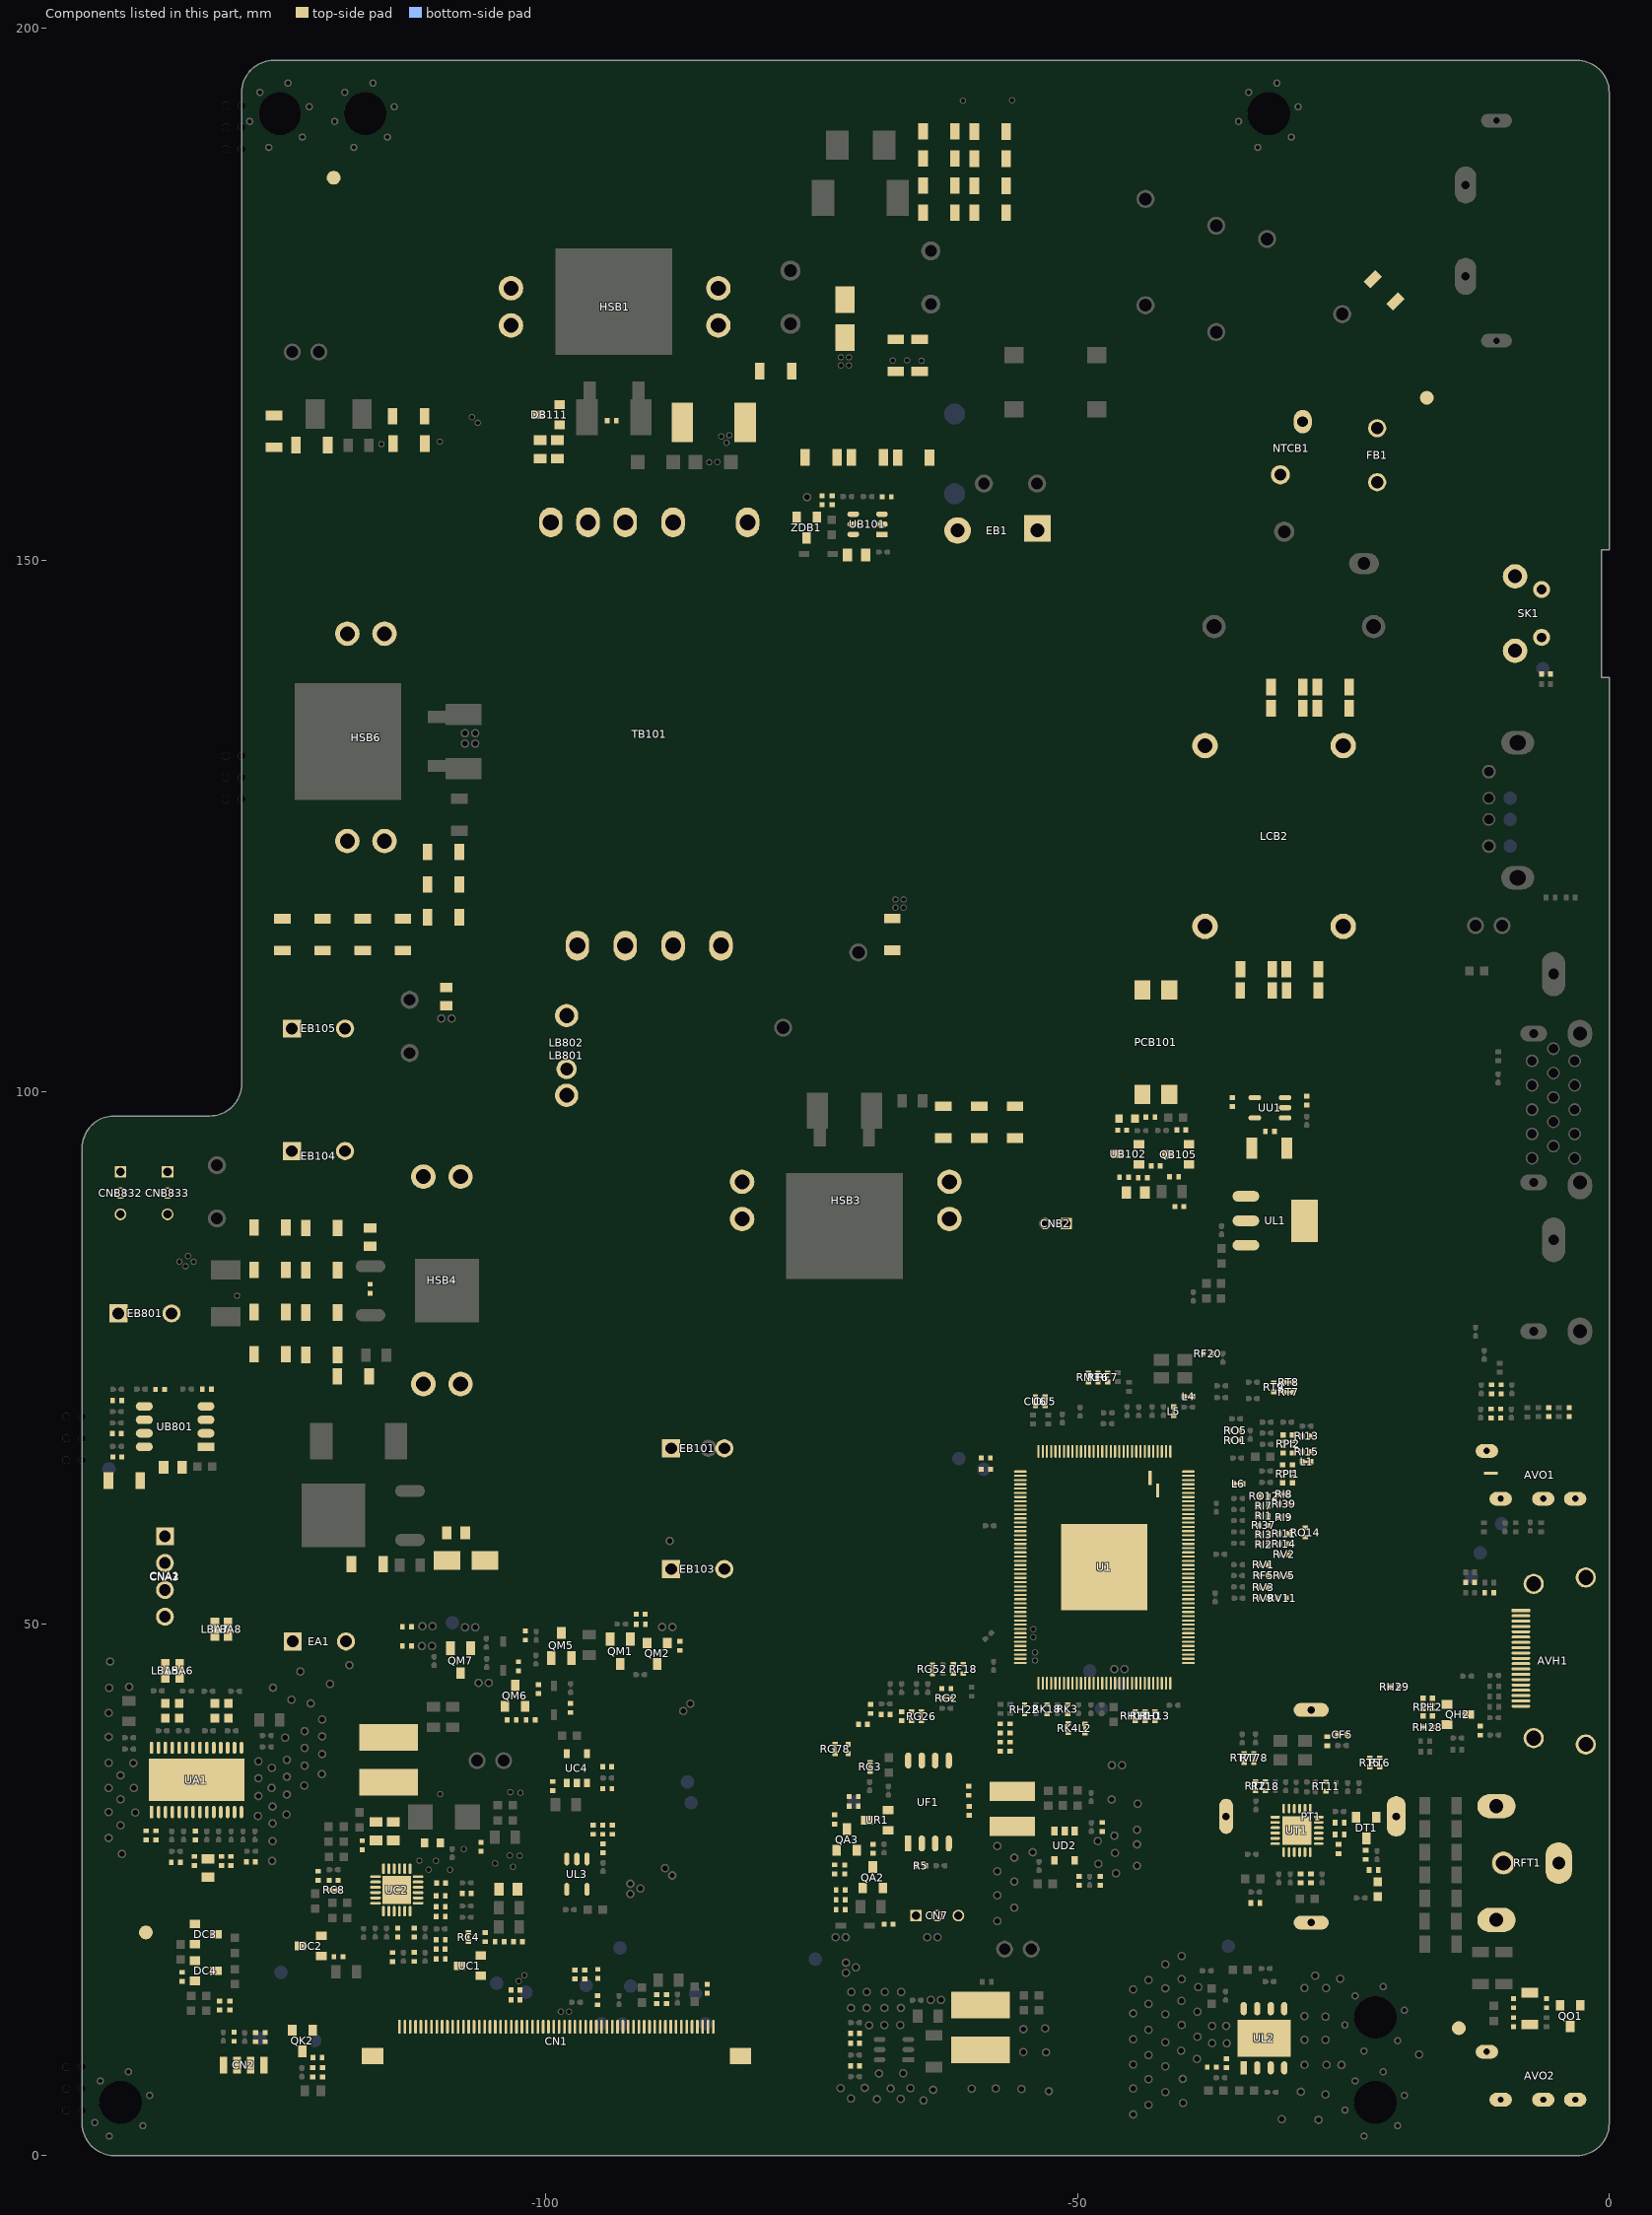
[diagram p0: the components of this part, seen from the top]
# Altium PCB MISC86383-9.PcbDoc (part 5 of 18)
Units mm, origin at the board's own origin, x right, y up, seen from the top; angles counter-clockwise.
Board outline 143.6 x 197 mm, 2 copper layers (TopLayer, BottomLayer), stack 1.571 mm thick; 743 components, 401 nets, 2996 pads, 1077 vias.
Unrouted connection lines stored in the file: 4.

## Footprints (in the part's own frame and the unit in brackets; to place one, negate y for a bottom-side part, rotate by r counter-clockwise, add the part's x,y. Pads: shape width x height; smd on the part's side, far side on the other; paste and mask are expansions set on the pad) (continued)
EC(10*12.5)-V-5#2 [mm] "机插5间距"
  round 0.5 on Keep-Out: 0(-0.75,0)
  rect 1.7x1.7 hole 1.1: 1(-2.5,0)
  rect 1.9x1.9 on Top Overlay: 1(-2.5,0)
  round 1.9 on Top Overlay: 1(2.5,0)
  round 1.7 hole 1.1: 2(2.5,0)
  BottomLayer lines w0.6: -2.92,-0.262 -2.89,-0.31 ; -2.92,-0.262 -2.991,-0.148 -4.056,1.556 ; -2.5,0 -2.627,0.127 -4.056,1.556 ; -2.19,0.39 -2.238,0.42 -2.42,0.534 -4.056,1.556 ; 2.19,-0.39 2.238,-0.42 ; 2.5,0 4.056,-1.556 ; 2.89,0.31 2.92,0.262 2.92,0.262 ; 2.238,-0.42 4.056,-1.556 ; 2.238,-0.42 2.238,-0.42 ; 2.238,-0.42 2.238,-0.42 ; 2.92,0.262 4.056,-1.556 ; 2.92,0.262 2.92,0.262
  silkscreen extent -5.2,-5.21 5.57,5.21, body extent -4.98,-4.99 5.01,4.99, height 14.01
EC(10*12.5)-V-5#3 [mm] "机插5间距"
  round 0.5 on Keep-Out: 0(-0.75,0)
  rect 1.7x1.7 hole 1.1: 1(-2.5,0)
  rect 1.9x1.9 on Top Overlay: 1(-2.5,0)
  round 1.9 on Top Overlay: 1(2.5,0)
  round 1.7 hole 1.1: 2(2.5,0)
  BottomLayer lines w0.6: -2.89,-0.31 -2.92,-0.262 -3.129,0.072 -4.056,1.556 ; -2.5,0 -2.78,0.28 -4.056,1.556 ; -2.19,0.39 -2.238,0.42 -2.5,0.584 -2.558,0.62 -2.754,0.742 -4.056,1.556 ; 2.19,-0.39 2.238,-0.42 ; 2.5,0 2.52,-0.02 2.704,-0.204 4.056,-1.556 ; 2.89,0.31 2.92,0.262 2.92,0.262 ; 2.238,-0.42 2.5,-0.584 2.52,-0.596 4.056,-1.556 ; 2.238,-0.42 2.238,-0.42 ; 2.238,-0.42 2.238,-0.42 ; 2.92,0.262 2.92,0.262 ; 2.92,0.262 3.016,0.108 4.056,-1.556
  silkscreen extent -5.2,-5.21 5.57,5.21, body extent -4.98,-4.99 5.01,4.99, height 14.01
EC(10*12.5)-V-5#4 [mm] "机插5间距"
  round 0.5 on Keep-Out: 0(0.025,-0.953)
  rect 1.7x1.7 hole 1.1: 1(-2.5,0)
  rect 1.9x1.9 on Top Overlay: 1(-2.5,0)
  round 1.9 on Top Overlay: 1(2.5,0)
  round 1.7 hole 1.1: 2(2.5,0)
  BottomLayer lines w0.6: -2.89,-0.31 -2.92,-0.262 -3.084,0 -4.056,1.556 ; -2.5,0 -4.056,1.556 ; -2.19,0.39 -2.238,0.42 -2.5,0.584 -4.056,1.556 ; 2.19,-0.39 2.238,-0.42 ; 2.5,0 4.056,-1.556 ; 2.89,0.31 2.92,0.262 2.92,0.262 ; 2.238,-0.42 4.056,-1.556 ; 2.238,-0.42 2.238,-0.42 ; 2.238,-0.42 2.238,-0.42 ; 2.92,0.262 4.056,-1.556 ; 2.92,0.262 2.92,0.262
  silkscreen extent -5.2,-5.21 5.57,5.21, body extent -4.98,-4.99 5.01,4.99, height 14.01
EC(10*12.5)-V-5#5 [mm] "机插5间距"
  round 0.5 on Keep-Out: 0(-0.75,0)
  rect 1.7x1.7 hole 1.1: 1(-2.5,0)
  rect 1.9x1.9 on Top Overlay: 1(-2.5,0)
  round 1.9 on Top Overlay: 1(2.5,0)
  round 1.7 hole 1.1: 2(2.5,0)
  BottomLayer lines w0.6: -2.89,-0.31 -2.92,-0.262 -3.182,0.157 -4.056,1.556 ; -2.5,0 -2.792,0.292 -4.056,1.556 ; -2.19,0.39 -2.238,0.42 -2.5,0.584 -4.056,1.556 ; 2.19,-0.39 2.238,-0.42 ; 2.5,0 4.056,-1.556 ; 2.89,0.31 2.92,0.262 2.92,0.262 ; 2.238,-0.42 4.056,-1.556 ; 2.238,-0.42 2.238,-0.42 ; 2.238,-0.42 2.238,-0.42 ; 2.92,0.262 4.056,-1.556 ; 2.92,0.262 2.92,0.262
  silkscreen extent -5.2,-5.21 5.57,5.21, body extent -4.98,-4.99 5.01,4.99, height 14.01
EC(10*12.5)-V-5#6 [mm] "机插5间距"
  round 0.5 on Keep-Out: 0(-0.75,0)
  rect 1.7x1.7 hole 1.1: 1(-2.5,0)
  rect 1.9x1.9 on Top Overlay: 1(-2.5,0)
  round 1.9 on Top Overlay: 1(2.5,0)
  round 1.7 hole 1.1: 2(2.5,0)
  BottomLayer lines w0.6: -2.89,-0.31 -2.92,-0.262 -3.084,0 -4.056,1.556 ; -2.5,0 -2.68,0.18 -4.056,1.556 ; -2.19,0.39 -2.238,0.42 -2.377,0.506 -2.5,0.584 -2.68,0.696 -4.056,1.556 ; 2.19,-0.39 2.238,-0.42 ; 2.5,0 4.056,-1.556 ; 2.89,0.31 2.92,0.262 2.92,0.262 ; 2.238,-0.42 4.056,-1.556 ; 2.238,-0.42 2.238,-0.42 ; 2.238,-0.42 2.238,-0.42 ; 2.92,0.262 4.056,-1.556 ; 2.92,0.262 2.92,0.262
  silkscreen extent -5.2,-5.21 5.57,5.21, body extent -4.98,-4.99 5.01,4.99, height 14.01
EC(18*36)-H7.5-1 [mm] "SAMXON  (18*36)"
  round 2.7 on Top Overlay: 1(-3.75,0)
  rect 2.5x2.5 hole 1.3 copper offset 0,0.2: 1(3.75,0)
  rect 2.7x2.7 on Top Overlay: 1(3.75,0)
  round 2.5 hole 1.3: 2(-3.75,0)
  KeepOutLayer lines w0.127: -6.75,-44 6.75,-44 6.75,-4.5 -6.75,-4.5 -6.75,-44
  silkscreen extent -9.5,-43.5 9.5,-1, body extent -9.09,-43.09 9.03,0.4, height 14.96
EVA(7*7*3) [mm] "7*7*3"
  silkscreen extent -4.5,-4.5 4.5,4.5
FFC60H/0.5S-11 [mm] "XFE,0.5-22-60PBX-P,翻盖打开高度4.62mm,0807_2018"
  rect 0.25x1.3 smd mask+0.051: 1(-14.75,1.375)
  oval 0.25x1.3 smd mask+0.051: 2(-14.25,1.375) 3(-13.75,1.375) 4(-13.25,1.375) 5(-12.75,1.375) 6(-12.25,1.375) 7(-11.75,1.375) 8(-11.25,1.375) 9(-10.75,1.375) 10(-10.25,1.375) 11(-9.75,1.375) 12(-9.25,1.375) 13(-8.75,1.375) 14(-8.25,1.375) 15(-7.75,1.375) 16(-7.25,1.375) 17(-6.75,1.375) 18(-6.25,1.375) 19(-5.75,1.375) 20(-5.25,1.375) 21(-4.75,1.375) 22(-4.25,1.375) 23(-3.75,1.375) 24(-3.25,1.375) 25(-2.75,1.375) 26(-2.25,1.375) 27(-1.75,1.375) 28(-1.25,1.375) 29(-0.75,1.375) 30(-0.25,1.375) 31(0.25,1.375) 32(0.75,1.375) 33(1.25,1.375) 34(1.75,1.375) 35(2.25,1.375) 36(2.75,1.375) 37(3.25,1.375) 38(3.75,1.375) 39(4.25,1.375) 40(4.75,1.375) 41(5.25,1.375) 42(5.75,1.375) 43(6.25,1.375) 44(6.75,1.375) 45(7.25,1.375) 46(7.75,1.375) 47(8.25,1.375) 48(8.75,1.375) 49(9.25,1.375) 50(9.75,1.375) 51(10.25,1.375) 52(10.75,1.375) 53(11.25,1.375) 54(11.75,1.375) 55(12.25,1.375) 56(12.75,1.375) 57(13.25,1.375) 58(13.75,1.375) 59(14.25,1.375) 60(14.75,1.375)
  rect 2x1.5 smd mask+0.051: 61(17.29,-1.375) 62(-17.29,-1.375)
  silkscreen extent -17.45,-3.88 17.45,3.5
Fixed [mm] "麦拉片塑胶固定柱(4.50×6.49mm-尼龙-白色)"
  round 2.5 on Keep-Out: 0(0,0)
  silkscreen extent -1.9,-1.9 1.9,1.9
FUSE1.1A-S [mm] "保险丝：FSMD005-1206(FUZETEC)（兼容1206F8.00A063V 高度0.8mm），18.03.07）"
  rect 1x2 smd: 1(-1.65,0) 2(1.65,0)
  silkscreen extent -2.4,-1.2 2.4,1.2, body extent -1.75,-0.9 1.75,0.9, height 1
"FUSE8.5*4-V-5(T3.15AL 250V~)" [mm] "SMT1315AP/2010T1A250VA1(编带/华德)"
  round 1.7 hole 1.15: 1(2.54,0) 2(-2.54,0)
  round 1.9 on Top Overlay: 4(2.54,0) 5(-2.54,0)
  BottomLayer lines w1: -2.312,0.271 -2.338,0.289 -2.568,0.451 -3.977,1.437 ; 2.811,0.228 2.829,0.202 2.942,0.041 2.971,0 3.113,-0.203 3.158,-0.267 3.173,-0.289 3.977,-1.437 ; -2.54,0 -2.712,0.172 -2.728,0.188 -3.977,1.437 ; 2.54,0 2.712,-0.172 3.977,-1.437 ; -2.811,-0.228 -2.829,-0.202 -2.942,-0.041 -2.953,-0.026 -2.971,0 -3.031,0.085 -3.099,0.183 -3.977,1.437 ; 2.312,-0.271 2.338,-0.289 2.568,-0.451 3.977,-1.437
  silkscreen extent -4.3,-2.1 4.3,2.1, body extent -4.3,-2.1 4.3,2.1, height 8.5
GND [mm] "导通线"
  rect 0.66x0.3 smd paste-0.45 mask-0.45: JP_1K(-0.32,0) JP_2K(0.32,0)
HDMI-HS-11 [mm] "客供；R-S151U-162;垫高；15.06.11(18.08.31 更新钢网）"
  rect 0.28x1.75 smd: 1(4.75,7.7)
  oval 0.28x1.75 smd: 2(4.25,7.7) 3(3.75,7.7) 4(3.25,7.7) 5(2.75,7.7) 6(2.25,7.7) 7(1.75,7.7) 8(1.25,7.7) 9(0.75,7.7) 10(0.25,7.7) 11(-0.25,7.7) 12(-0.75,7.7) 13(-1.25,7.7) 14(-1.75,7.7) 15(-2.25,7.7) 16(-2.75,7.7) 17(-3.25,7.7) 18(-3.75,7.7) 19(-4.25,7.7)
  rect 3x4 on Top Paste: 4(-7.45,2.3) 4(-7.25,6.6) 4(7.25,6.6) 4(7.45,2.3)
  round 1.9 hole 1.4 mask+0.076: 20(-7.25,6.5) 21(-7.85,1.6) 22(7.85,1.6) 23(7.25,6.5)
  silkscreen extent -7.5,-0.02 7.5,8.41, body extent -10.25,-81.2 10.25,9.06, height 12.13
"Heat-Shrinkable Tube" [mm] "收缩前壁厚0.3+-0.05，收缩后壁厚0.6+-0.1"
  round 0.3 on Mech2: 0(0,0)
"High Voltage" [mm]
  silkscreen extent -0.53,-1.52 0.43,1.27
HS151 [mm] "铝,本色,20x14x5.8mm.11/1/2019"
  round 2.5 on Top Overlay: 0(-9.75,-1.75) 0(-9.75,1.75) 0(9.75,-1.75) 0(9.75,1.75)
  round 2.3 hole 1.4: 1(-9.75,1.75) 2(-9.75,-1.75) 3(9.75,-1.75) 4(9.75,1.75)
  silkscreen extent -10.03,-2.93 10.03,2.93
HS(15X15X5)-S [mm] "YT.YT-P-151505.2019/9/18"
  silkscreen extent -7.63,-7.63 7.63,7.63, body extent -7.5,-7.5 7.5,7.5, height 5
HS(18.8*13.8*5) [mm] "18.8×13.8×5-本色-THD;14.10.21"
  silkscreen extent -7,-9.5 7,9.5
KEY-HD-6 [mm] "春生KFC-A06--E-4-160-7.5/4; 中心高度为4mm;14.09.04;171102修正突出距离(12/9/2019增加3D)"
  round 2.5 on Top Overlay: 0(-3.5,5) 0(3.5,5)
  round 1.8 on Top Overlay: 0(-2.25,2.5) 0(2.25,2.5)
  round 1.6 hole 0.9: 1(2.25,2.5) 2(-2.25,2.5)
  round 2.286 hole 1.3: 3(3.5,5) 4(-3.5,5)
  silkscreen extent -3.85,0 3.85,6.6, body extent -4.22,-4.05 4.22,6.2, height 7
L0402 [mm] "电感"
  rect 0.45x0.55 smd mask+0.076: 1(-0.425,0) 2(0.425,0)
  silkscreen extent -0.8,-0.42 0.8,0.43, body extent -0.5,-0.25 0.5,0.25, height 0.5
L0603 [mm] "片式磁珠、电感、ESD"
  rect 0.813x0.8 smd mask+0.076: 1(-0.706,0) 2(0.706,0)
  silkscreen extent -1.27,-0.55 1.27,0.55, body extent -0.8,-0.4 0.8,0.4, height 0.8
L(4*3*2.55)-S [mm] "贴片磁珠；SMB -302540-K5B- L1;15.02.05（17.12.07更新高度信息）"
  rect 2.5x1.8 smd: 1(-1.775,0) 2(1.775,0)
  silkscreen extent -2.12,-1.6 2.12,1.6, body extent -2.55,-1.6 2.55,1.6, height 2.7
L(4.5*3.5)-S [mm] "SMD4532-6R8M-023"
  rect 1.8x4.3 smd: 1(-1.65,0) 2(1.65,0)
  TopLayer pour cut-out: -0.76,2.15 0.796,2.15 0.796,2.141 0.796,-2.149 -0.756,-2.149 -0.756,-2.15
  silkscreen extent -2.83,-2.44 3.3,2.44
L(5.8*4.5)-S [mm] "APC52A45M4R7\电感\Cailank;170317更新阻焊兼容L(4*3.0)-S"
  rect 2.5x5.5 smd paste-5.5: 1(2.105,0) 2(-2.105,0)
  TopLayer pour cut-out: -0.849,2.746 -0.845,2.75 0.861,2.75 0.861,-2.749 0.861,-2.753 0.859,-2.753 -0.862,-2.753
  silkscreen extent -1.5,-2.9 3.88,2.9, body extent -3.05,-2.65 3.07,2.74, height 4.8
L(13.5*15.5)-V-5 [mm] "深圳秀益达；SA-A048-036-A SPK1214RBL-680K；14.11.19"
  round 1.9 hole 1.2 mask+0.076: 1(-2.5,0) 2(2.5,0)
  round 2.1 on Top Overlay mask+0.076: 3(-2.5,0) 4(2.5,0)
  silkscreen extent -6.75,-6.75 6.75,6.75, body extent -6.72,-6.73 6.72,6.75, height 15.5
L/LC2/15*14.5-V7.5 [mm] "SYDR1212-L003-YMX"
  round 2.2 hole 1.4: 1(-3.75,0) 2(3.75,0)
  round 2.4 on Top Overlay: 1(-3.75,0) 1(3.75,0)
  silkscreen extent -7.25,-7.25 7.25,7.25
L/LC4/21*17-H-17*13 [mm] "CH,SQ1614-10.5mH,1206_2018"
  round 2.6 on Top Overlay mask+0.076: 0(-8.5,-6.5) 0(-8.5,6.5) 0(8.5,6.5) 0(8.5,-6.5)
  round 2.4 hole 1.4 mask+0.076: 1(-8.5,-6.5) 2(8.5,-6.5) 3(8.5,6.5) 4(-8.5,6.5)
  silkscreen extent -10.5,-8.5 10.5,8.5, body extent -10.5,-8.5 10.5,8.5, height 13.99
Manufacture_Info [mm]
  round 0.3 on Mech2: 0(0,0)
MARK [mm] "SMD 使用"
  round 1.3 smd paste+0 mask+0.65: 0(0,0)
  TopLayer circle w0.254: c0,0 r1.444
  TopLayer pour cut-out: -1.3,0 -1.201,-0.497 -0.919,-0.919 -0.497,-1.201 0,-1.3 0,-1.3 0.497,-1.201 0.919,-0.919 1.201,-0.497 1.3,0 1.3,0 1.201,0.497 0.919,0.919 0.497,1.201 0,1.3 0,1.3 -0.497,1.201 -0.919,0.919 -1.201,0.497 -1.3,0
Mylar [mm] "180×180×0.4mm-PC-黑色"
"NO DOLBY-SILK" [mm]
  silkscreen extent -0.4,-4.5 36.6,5
NTC(10*5)-V5 [mm] "热敏电阻 SCK152R58MSY  (为勤电子）;161022更新椭圆孔"
  round 1.8 hole 1.1: 1(-2.5,1.05)
  round 2 on Top Overlay: 2(-2.5,1.05)
  oval 2.2x1.7 hole 1 slot 1.5 at 0 deg: 2(2.5,-1.05)
  oval 2.4x1.9 on Top Overlay: 3(2.5,-1.05)
  silkscreen extent -5.77,-2.5 5.77,2.5, body extent -5.75,-2 5.75,2, height 13.75
OC4-S-1 [mm] "巨路国际；肖特基LTV-817S-TA-B"
  rect 1.5x1.8 smd: 1(-1.27,-4.9) 2(1.27,-4.9) 3(1.27,4.9) 4(-1.27,4.9)
  silkscreen extent -3.17,-5.35 2.55,3.5, body extent -2.3,-5.08 2.3,5.08, height 3.88
PCB_NAME [mm]
  round 0.3 on Mech2: 0(0,0)
PCB_TIME [mm]
  round 0.3 on Mech2: 0(0,0)
PHONE-HD-43 [mm] "乐友；CK3-3.5-03C;160624"
  oval 1.5x2.3 on Top Overlay: 0(-2.25,10.2) 0(-2.25,3.2) 0(-2.25,6.2) 0(2.25,11.5)
  round 1.1 on Keep-Out: 0(0,8.5) 0(0,1.5)
  oval 1.3x2.1 hole 0.6 slot 1.4 at 90 deg: 1(2.25,11.5) 2(-2.25,10.2) 3(-2.25,3.2) 4(-2.25,6.2)
  silkscreen extent -3.1,0 3.1,12.7
QFN24/0.5-3 [mm] "R620D(Rafael Micro)，修改EPAD焊盘/CY8C4014LQI-422(0.6mm)"
  oval 0.9x0.26 smd: 1(-2.05,1.25) 2(-2.05,0.75) 3(-2.05,0.25) 4(-2.05,-0.25) 5(-2.05,-0.75) 6(-2.05,-1.25) 13(2.05,-1.25) 14(2.05,-0.75) 15(2.05,-0.25) 16(2.05,0.25) 17(2.05,0.75) 18(2.05,1.25)
  oval 0.26x0.9 smd: 7(-1.25,-2.05) 8(-0.75,-2.05) 9(-0.25,-2.05) 10(0.25,-2.05) 11(0.75,-2.05) 12(1.25,-2.05) 19(1.25,2.05) 20(0.75,2.05) 21(0.25,2.05) 22(-0.25,2.05) 23(-0.75,2.05) 24(-1.25,2.05)
  rect 2.7x2.7 smd paste-2 mask-2: 25(0,0)
  silkscreen extent -3.28,-3.33 3.21,3.35, body extent -2.08,-2.07 2.07,2.07, height 1
QFN24/0.5-5 [mm] "BEKEN ,     BK2433;BQ24196(1mm)"
  oval 1x0.27 smd: 1(-2,1.25) 2(-2,0.75) 3(-2,0.25) 4(-2,-0.25) 5(-2,-0.75) 6(-2,-1.25) 13(2,-1.25) 14(2,-0.75) 15(2,-0.25) 16(2,0.25) 17(2,0.75) 18(2,1.25)
  oval 0.27x1 smd: 7(-1.25,-2) 8(-0.75,-2) 9(-0.25,-2) 10(0.25,-2) 11(0.75,-2) 12(1.25,-2) 19(1.25,2) 20(0.75,2) 21(0.25,2) 22(-0.25,2) 23(-0.75,2) 24(-1.25,2)
  rect 2.667x2.667 smd paste-0.6 mask-0.6: 25(0,0)
  silkscreen extent -3.38,-3.5 3.1,3.5, body extent -2.05,-2.05 2.05,2.05, height 1
QFP156/0.4-2 [mm] "Mstar,MSD3393LB"
  oval 0.2x1.2 smd: 1(-9,-7.9) 2(-8.6,-7.9) 3(-8.2,-7.9) 4(-7.8,-7.9) 5(-7.4,-7.9) 6(-7,-7.9) 7(-6.6,-7.9) 8(-6.2,-7.9) 9(-5.8,-7.9) 10(-5.4,-7.9) 11(-5,-7.9) 12(-4.6,-7.9) 13(-4.2,-7.9) 14(-3.8,-7.9) 15(-3.4,-7.9) 16(-3,-7.9) 17(-2.6,-7.9) 18(-2.2,-7.9) 19(-1.8,-7.9) 20(-1.4,-7.9) 21(-1,-7.9) 22(-0.6,-7.9) 23(-0.2,-7.9) 24(0.2,-7.9) 25(0.6,-7.9) 26(1,-7.9) 27(1.4,-7.9) 28(1.8,-7.9) 29(2.2,-7.9) 30(2.6,-7.9) 31(3,-7.9) 32(3.4,-7.9) 33(3.8,-7.9) 34(4.2,-7.9) 35(4.6,-7.9) 36(5,-7.9) 37(5.4,-7.9) 38(5.8,-7.9) 39(6.2,-7.9) 40(6.6,-7.9) 41(7,-7.9) 42(7.4,-7.9) 43(7.8,-7.9) 44(8.2,-7.9) 45(8.6,-7.9) 46(9,-7.9) 79(9,7.9) 80(8.6,7.9) 81(8.2,7.9) 82(7.8,7.9) 83(7.4,7.9) 84(7,7.9) 85(6.6,7.9) 86(6.2,7.9) 87(5.8,7.9) 88(5.4,7.9) 89(5,7.9) 90(4.6,7.9) 91(4.2,7.9) 92(3.8,7.9) 93(3.4,7.9) 94(3,7.9) 95(2.6,7.9) 96(2.2,7.9) 97(1.8,7.9) 98(1.4,7.9) 99(1,7.9) 100(0.6,7.9) 101(0.2,7.9) 102(-0.2,7.9) 103(-0.6,7.9) 104(-1,7.9) 105(-1.4,7.9) 106(-1.8,7.9) 107(-2.2,7.9) 108(-2.6,7.9) 109(-3,7.9) 110(-3.4,7.9) 111(-3.8,7.9) 112(-4.2,7.9) 113(-4.6,7.9) 114(-5,7.9) 115(-5.4,7.9) 116(-5.8,7.9) 117(-6.2,7.9) 118(-6.6,7.9) 119(-7,7.9) 120(-7.4,7.9) 121(-7.8,7.9) 122(-8.2,7.9) 123(-8.6,7.9) 124(-9,7.9)
  oct 2.5x2.15 on Top Paste: 1(-2.8,-2.45) 1(-2.8,0) 1(-2.8,2.45) 1(0,-2.45) 1(0,0) 1(0,2.45) 1(2.8,-2.45) 1(2.8,0) 1(2.8,2.45)
  oct 2.5x2.15 on Top Solder: 1(-2.8,-2.45) 1(-2.8,0) 1(-2.8,2.45) 1(0,-2.45) 1(0,0) 1(0,2.45) 1(2.8,-2.45) 1(2.8,0) 1(2.8,2.45)
  oval 1.2x0.2 smd: 47(10.9,-6.2) 48(10.9,-5.8) 49(10.9,-5.4) 50(10.9,-5) 51(10.9,-4.6) 52(10.9,-4.2) 53(10.9,-3.8) 54(10.9,-3.4) 55(10.9,-3) 56(10.9,-2.6) 57(10.9,-2.2) 58(10.9,-1.8) 59(10.9,-1.4) 60(10.9,-1) 61(10.9,-0.6) 62(10.9,-0.2) 63(10.9,0.2) 64(10.9,0.6) 65(10.9,1) 66(10.9,1.4) 67(10.9,1.8) 68(10.9,2.2) 69(10.9,2.6) 70(10.9,3) 71(10.9,3.4) 72(10.9,3.8) 73(10.9,4.2) 74(10.9,4.6) 75(10.9,5) 76(10.9,5.4) 77(10.9,5.8) 78(10.9,6.2) 125(-10.9,6.2) 126(-10.9,5.8) 127(-10.9,5.4) 128(-10.9,5) 129(-10.9,4.6) 130(-10.9,4.2) 131(-10.9,3.8) 132(-10.9,3.4) 133(-10.9,3) 134(-10.9,2.6) 135(-10.9,2.2) 136(-10.9,1.8) 137(-10.9,1.4) 138(-10.9,1) 139(-10.9,0.6) 140(-10.9,0.2) 141(-10.9,-0.2) 142(-10.9,-0.6) 143(-10.9,-1) 144(-10.9,-1.4) 145(-10.9,-1.8) 146(-10.9,-2.2) 147(-10.9,-2.6) 148(-10.9,-3) 149(-10.9,-3.4) 150(-10.9,-3.8) 151(-10.9,-4.2) 152(-10.9,-4.6) 153(-10.9,-5) 154(-10.9,-5.4) 155(-10.9,-5.8) 156(-10.9,-6.2)
  rect 8.1x8.1 smd paste-8.1 mask-8.1: 157(0,0)
  silkscreen extent -12.7,-9.87 12.7,9.69, body extent -10.1,-7.1 10.1,7.1, height 1.6
R0402#1 [mm] "片式电阻"
  rect 0.45x0.5 smd mask+0.076: 1(-0.425,0) 2(0.425,0)
  silkscreen extent -0.8,-0.4 0.8,0.4, body extent -0.5,-0.25 0.5,0.25, height 0.5
R0402#2 [mm] "片式电阻"
  rect 0.45x0.5 smd mask+0.076: 1(-0.425,0) 1(-0.425,0) 2(0.425,0) 2(0.425,0)
  silkscreen extent -0.8,-0.4 0.8,0.4, body extent -0.5,-0.25 0.5,0.25, height 0.5
R0402SC [mm]
  rect 0.45x0.5 smd mask+0.076: 1(-0.425,0) 2(0.425,0)
  rect 0.42x0.25 smd paste-0.5 mask-0.5: 3(0,0)
  silkscreen extent -0.8,-0.4 0.8,0.4, body extent -0.5,-0.25 0.5,0.25, height 0.5
R0603 [mm] "贴片电阻"
  rect 0.7x0.8 smd mask+0.076: 1(-0.756,0) 2(0.756,0)
  silkscreen extent -1.25,-0.54 1.25,0.54, body extent -0.8,-0.4 0.8,0.4, height 0.8
R0603SC [mm] "贴片电阻(12/13/2019增大中间焊盘的大小)"
  rect 0.7x0.8 smd mask+0.076: 1(-0.756,0) 2(0.756,0)
  rect 0.9x0.8 smd paste-0.5 mask-0.5: 3(0,0)
  silkscreen extent -1.25,-0.54 1.25,0.54, body extent -0.8,-0.4 0.8,0.4, height 0.8
R0805 [mm] "贴片电阻"
  rect 0.9x1.2 smd mask+0.076: 1(-0.866,0) 2(0.866,0)
  silkscreen extent -1.47,-0.75 1.47,0.75, body extent -1,-0.63 1,0.62, height 0.5
R1206 [mm] "贴片电阻"
  rect 0.9x1.55 smd mask+0.076: 1(-1.5,0) 2(1.5,0)
  silkscreen extent -2.1,-0.93 2.1,0.93, body extent -1.6,-0.8 1.6,0.8, height 0.55
R2512-1 [mm] "PSA;Size 2512 2W;16.01.20(17.06.19修改焊盘大小，增强爬锡，解决浮高问题）"
  rect 2x3.7 smd: 1(-2.95,0) 2(2.95,0)
  silkscreen extent -3.3,-2 3.3,2, body extent -3.25,-1.65 3.25,1.65, height 0.75
RA0402 [mm] "排阻"
  rect 0.5x0.5 smd mask+0.076: 1(-0.45,0.85) 2(0.45,0.85) 7(-0.45,-0.85) 8(0.45,-0.85)
  rect 0.5x0.3 smd mask+0.076: 3(-0.45,0.25) 4(0.45,0.25) 5(-0.45,-0.25) 6(0.45,-0.25)
  silkscreen extent -0.85,-1.27 0.85,1.27, body extent -0.51,-1 0.51,1, height 0.35
REMOTE-HS-1 [mm] "vishay;HS75438D;侧卧贴；14.09.03"
  rect 0.7x1.6 smd mask+0.076: 1(-1.905,2.275) 2(-0.635,2.275) 3(0.635,2.275) 4(1.905,2.275)
  silkscreen extent -3.47,-0.7 3.47,2.65
SHIELD(16*20*6) [mm] "屏蔽罩：用于与高频头分离的做法"
  oval 2.1x4.1 on Top Overlay: 0(-8,10) 0(8,10)
  oval 4.1x2.1 on Top Overlay: 0(0,0) 0(0,20)
  oval 3.3x1.3 hole 0.7 slot 2.7 at 0 deg: 1(0,0) 3(0,20)
  oval 1.8x3.8 hole 0.7 slot 2.7 at 90 deg: 2(8,10)
  oval 1.3x3.3 hole 0.7 slot 2.7 at 90 deg: 4(-8,10)
  silkscreen extent -9,-1 9,21, body extent -8.57,-0.15 8.57,20.15, height 6
"Silica gel-10" [mm] "硅胶"
  silkscreen extent -3,-5 3,5
"Silica gel-20" [mm] "硅胶"
  silkscreen extent -3,-10 3,10
SIP2/2.0D-1 [mm] "捷仕泰/铭锋达"
  rect 1.3x1.3 on Top Overlay: 0(-1,0)
  round 1.3 on Top Overlay: 0(1,0)
  rect 1.1x1.1 hole 0.8: 1(-1,0)
  round 1.1 hole 0.8: 2(1,0)
  silkscreen extent -3,-3.2 3,1.8, body extent -3,-3.2 3,1.8, height 6
SIP3/2.0D-3 [mm] "捷仕泰   A2004-03-A1MA-P,插线高度11mm"
  rect 1.5x1.5 on Top Overlay: 0(-2,0)
  round 1.5 on Top Overlay: 0(0,0) 0(2,0)
  rect 1.1x1.1 hole 0.8: 1(-2,0)
  round 1.1 hole 0.8: 2(0,0) 3(2,0)
  silkscreen extent -4,-2.13 4,3.07, body extent -4,-2.18 4,3.1, height 7.8
SIP3/2.0D-CP [mm] "捷仕泰/铭锋达;带扣插座与非带扣插座 兼容；15.07.11"
  rect 1.4x1.4 on Top Overlay: 0(-2,0)
  round 1.4 on Top Overlay: 0(0,0) 0(2,0)
  rect 1.1x1.1 hole 0.8: 1(-2,0)
  round 1.1 hole 0.8: 2(0,0) 3(2,0)
  silkscreen extent -4,-3.2 4,3.07, body extent -4,-3.2 4,1.8, height 6
SIP3H/2.0D-3 [mm] "捷仕泰：A2004AW-03-A1MA-P，带扣，加强筋"
  rect 1.6x1.6 on Top Overlay: 0(-2,0)
  round 1.6 on Top Overlay: 0(0,0) 0(2,0)
  rect 1.1x1.1 hole 0.8: 1(-2,0)
  round 1.1 hole 0.8: 2(0,0) 3(2,0)
  silkscreen extent -4.1,-7.95 4.1,1.5
SIP4/2.5D-2 [mm] "捷仕泰，A2502-04-A5WA-P（为保证与SIP4/2.54D-1兼容。改PIN间距为2.52mm，18.05.28）"
  rect 1.905x1.905 on Top Overlay: 0(-3.78,0)
  round 1.905 on Top Overlay: 0(-1.26,0) 0(1.26,0) 0(3.78,0)
  rect 1.651x1.651 hole 1.05: 1(-3.78,0)
  round 1.651 hole 1.05: 2(-1.26,0) 3(1.26,0) 4(3.78,0)
  silkscreen extent -6.4,-3.6 6.4,3
SIP4/2.54D-1 [mm] "捷仕泰/铭锋达"
  rect 1.905x1.905 on Top Overlay: 0(-3.78,0)
  round 1.905 on Top Overlay: 0(-1.26,0) 0(1.26,0) 0(3.78,0)
  rect 1.651x1.651 hole 1.05: 1(-3.78,0)
  round 1.651 hole 1.05: 2(-1.26,0) 3(1.26,0) 4(3.78,0)
  silkscreen extent -6.44,-3.5 6.44,2.5, body extent -6.35,-3.5 6.35,2.5, height 7
SIP4H/2.5D-7 [mm] "AMA,TJC3B-4AW,带扣、台阶。17.08.28"
  rect 1.85x1.85 on Top Overlay: 0(-3.75,0.18)
  round 1.85 on Top Overlay: 0(-1.25,0.18) 0(1.25,0.18) 0(3.75,0.18)
  rect 1.65x1.65 hole 1.05: 1(-3.75,0.18)
  round 1.65 hole 1.05: 2(-1.25,0.18) 3(1.25,0.18) 4(3.75,0.18)
  silkscreen extent -6.38,-7.35 6.38,1.91
SO-8A [mm] "FLASH"
  rect 1.6x0.8 smd: 1(-2.9,1.905)
  oval 1.6x0.8 smd: 2(-2.9,0.635) 3(-2.9,-0.635) 4(-2.9,-1.905) 5(2.9,-1.905) 6(2.9,-0.635) 7(2.9,0.635) 8(2.9,1.905)
  silkscreen extent -4.87,-2.54 2,3.43, body extent -3.1,-2.5 3.1,2.5, height 1.76
SO-23 [mm] "双向二极管封装"
  rect 0.8x1 smd: 1(0.953,1.016) 3(-0.952,1.016)
  rect 0.8x1.1 smd: 2(0,-0.966)
  silkscreen extent -1.55,-0.86 1.55,0.36, body extent -1.5,-1.25 1.5,1.25, height 1.1
SO-23-1 [mm] "双向二极管封装，小型"
  rect 0.8x1 smd: 1(-0.953,-1.016) 2(0.953,-1.016)
  rect 0.8x1.1 smd: 3(0,0.966)
  silkscreen extent -1.55,-0.36 1.55,0.86, body extent -1.5,-1.25 1.5,1.25, height 1.1
SOIC8 [mm] "W25X40BVSNIG/GD25Q32BSIG/GD25LQ16"
  rect 1.5x0.6 smd: 1(-3.9,1.905)
  oval 1.5x0.6 smd: 2(-3.9,0.635) 3(-3.9,-0.635) 4(-3.9,-1.905) 5(3.9,-1.905) 6(3.9,-0.635) 7(3.9,0.635) 8(3.9,1.905)
  silkscreen extent -5.71,-2.65 2.7,2.65, body extent -4.05,-2.69 4.05,2.69, height 2.17
SOP8/1.27-3 [mm] "LEADCHIP;LC1118;14-05-09"
  rect 1.238x0.6 smd: 1(-2.782,1.905)
  oval 1.238x0.6 smd: 2(-2.783,0.635) 3(-2.783,-0.635) 4(-2.782,-1.905) 5(2.782,-1.905) 6(2.783,-0.635) 7(2.783,0.635) 8(2.782,1.905)
  rect 3.5x5 smd paste-3 mask-3: EPAD(0,0)
  silkscreen extent -4.27,-2.5 4.16,3.37, body extent -3.1,-2.5 3.1,2.5, height 1.76
SOP23-5-1 [mm] "TI ,TLV70033-Q1  (WL2851E33-5/TR  高度1.25mm）"
  oval 0.5x1.2 smd: 1(-0.95,-1.425) 2(0,-1.425) 3(0.95,-1.425) 4(0.95,1.425) 5(-0.95,1.425)
  silkscreen extent -1.53,-3.12 1.52,0.88, body extent -1.53,-0.87 1.52,0.88, height 1.1
SOT-23 [mm]
  rect 0.8x1 smd: B(0.952,1.016) E(-0.953,1.016)
  rect 0.8x1.1 smd: C(-0.013,-0.966)
  silkscreen extent -1.55,-0.81 1.55,0.36, body extent -1.5,-1.25 1.5,1.25, height 1.1
SOT-23-1 [mm]
  rect 0.8x1.1 smd: D(0,-1.15)
  rect 0.8x1.27 smd: G(0.95,1.2) S(-0.95,1.2)
  TopLayer pour cut-out: -1.583,0.903 -1.583,-0.905 1.587,-0.905 1.587,0.903
  silkscreen extent -1.55,-1.05 1.55,0.33, body extent -1.52,-1.48 1.52,1.48, height 1.25
SOT-23-5 [mm] "LPW5206(1.295mm)"
  rect 0.6x0.8 smd: 1(-0.95,-1.375) 2(0,-1.375) 3(0.95,-1.375) 4(0.95,1.375) 5(-0.95,1.375)
  silkscreen extent -1.5,-2.49 1.5,0.85, body extent -1.5,-0.85 1.5,0.85, height 1.45
SOT-23-RAK [mm] "TL431G-AE2-R(UTC)"
  rect 0.8x1.1 smd: A(0.013,0.966)
  rect 0.8x1 smd: K(0.953,-1.016) R(-0.953,-1.016)
  silkscreen extent -1.52,-0.36 1.52,0.86, body extent -1.5,-1.25 1.5,1.25, height 1.1
SOT-26 [mm] "LD7536R"
  rect 0.5x1.1 smd: 1(0.95,1.35)
  oval 0.5x1.1 smd: 2(0,1.35) 3(-0.95,1.35) 4(-0.95,-1.35) 5(0,-1.35) 6(0.95,-1.35)
  silkscreen extent -1.55,-2.54 1.55,2.9, body extent -1.55,-0.9 1.55,0.9, height 1.45
SOT-223 [mm]
  oval 1x2.5 smd: 1(-2.3,-2.75) 2(0,-2.75) 3(2.3,-2.75)
  rect 4x2.5 smd: 4(0,2.75)
  TopLayer pour cut-out: 2.3,-1.188 2.3,-4.312 -2.345,-4.312 -2.64,-4.253 -2.891,-4.086 -3.058,-3.835 -3.117,-3.54 -3.117,-3.54 -2.299,-3.54 -2.299,-1.956 -3.124,-1.956 -3.066,-1.662 -2.899,-1.413 -2.65,-1.247 -2.356,-1.188 -2.356,-1.188
  silkscreen extent -3.45,-2.75 3.45,2.81, body extent -3.35,-3.3 3.35,3.4, height 1.7
SSOP28/0.65-5 [mm] "TI;TPA3140D2PWPR;15.07.08"
  rect 1.15x0.34 smd mask+0.076: 1(-3.025,4.225)
  oval 1.15x0.34 smd mask+0.076: 2(-3.025,3.575) 3(-3.025,2.925) 4(-3.025,2.275) 5(-3.025,1.625) 6(-3.025,0.975) 7(-3.025,0.325) 8(-3.025,-0.325) 9(-3.025,-0.975) 10(-3.025,-1.625) 11(-3.025,-2.275) 12(-3.025,-2.925) 13(-3.025,-3.575) 14(-3.025,-4.225) 15(3.025,-4.225) 16(3.025,-3.575) 17(3.025,-2.925) 18(3.025,-2.275) 19(3.025,-1.625) 20(3.025,-0.975) 21(3.025,-0.325) 22(3.025,0.325) 23(3.025,0.975) 24(3.025,1.625) 25(3.025,2.275) 26(3.025,2.925) 27(3.025,3.575) 28(3.025,4.225)
  oct 1.05x1.318 on Top Paste mask+0.076: EPAD(-0.675,2.427) EPAD(-0.675,0.809) EPAD(-0.675,-0.809) EPAD(-0.675,-2.427) EPAD(0.675,2.427) EPAD(0.675,0.809) EPAD(0.675,-0.809) EPAD(0.675,-2.427)
  oct 1.05x1.318 on Top Solder mask+0.076: EPAD(-0.675,2.427) EPAD(-0.675,0.809) EPAD(-0.675,-0.809) EPAD(-0.675,-2.427) EPAD(0.675,2.427) EPAD(0.675,0.809) EPAD(0.675,-0.809) EPAD(0.675,-2.427)
  rect 4x9 smd paste-5 mask-5: EPAD(0,0)
  silkscreen extent -4.65,-4.9 4.64,4.9, body extent -2.25,-4.9 2.25,4.9, height 1.2
T-13.2×12.4×7.7-F14.5 [mm] "LHD;13.2×12.4×7.7-F14.5 中心出口高度6.3mm；160713(18.08.30 优化短槽孔）(19.03.11,优化地孔与IEC一致）"
  oval 2.5x3.8 on Top Overlay paste-4 mask-4: 0(-5.35,6.1) 0(5.35,6.1)
  round 2.3 on Top Overlay: 0(0,5.45)
  oval 4.1x2.7 on Top Overlay paste-4 mask-4: 0(0,0.25)
  round 2.1 hole 1.4: 1(0,5.45)
  oval 2.3x3.6 hole 1.3 slot 2.6 at 90 deg: 2(-5.35,6.1) 4(5.35,6.1)
  oval 3.9x2.5 hole 1.2 slot 2.6 at 0 deg: 3(0,0.25)
  KeepOutLayer pour cut-out: -1.438,5.45 -1.329,4.902 -1.019,4.438 -0.555,4.128 -0.007,4.019 -0.007,4.019 0.541,4.128 1.005,4.438 1.315,4.902 1.424,5.45 1.424,5.45 1.315,5.998 1.005,6.462 0.541,6.772 -0.007,6.881 -0.007,6.881 -0.555,6.772 -1.019,6.462 -1.329,5.998 -1.438,5.45
  silkscreen extent -6.3,0 6.3,7.9, body extent -7.55,-35.2 7.55,7.7, height 13.85
T/EQ2612*10 [mm] "SQ,SYEQ2613Z-T012033A,磁芯规格:EQ2612,0925_2018"
  oval 3x2.4 on Top Overlay: 0(-22.3,9.25) 0(-22.3,-5.75) 0(-22.3,-2.25) 0(-22.3,2.25) 0(-22.3,-9.25) 0(17.5,-6.75) 0(17.5,-2.25) 0(17.5,2.25) 0(17.5,6.75)
  oval 2.8x2.2 hole 1.5 mask+0.051: 1(-22.3,9.25) 3(-22.3,2.25) 4(-22.3,-2.25) 5(-22.3,-5.75) 6(-22.3,-9.25) 7(17.5,-6.75) 8(17.5,-2.25) 9(17.5,2.25) 10(17.5,6.75)
  silkscreen extent -23.77,-14.25 18.95,14.25